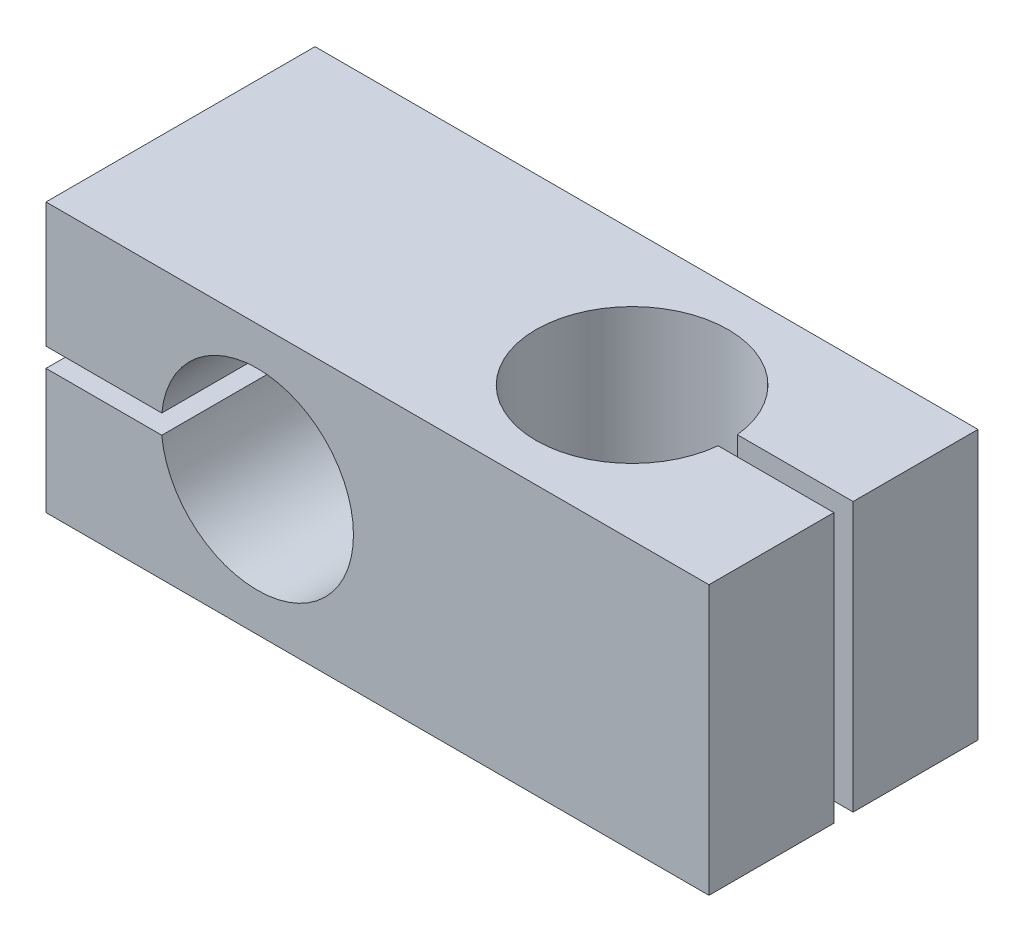
SolidWorks part; units mm, degrees
material "厂家标准"
ref_plane "前视基准面" through (0, 0, 0) normal (0, 0, 1) x (1, 0, 0)
ref_plane "上视基准面" through (0, 0, 0) normal (0, 1, 0) x (1, 0, 0)
ref_plane "右视基准面" through (0, 0, 0) normal (1, 0, 0) x (0, 0, -1)
sketch "草图1" plane through (0, 0, 0) normal (0, 0, 1) x (1, 0, 0)
  line L1 (-34.5, 14) -> (34.5, 14)
  line L2 (-34.5, 14) -> (-34.5, -14)
  line L3 (-34.5, -14) -> (34.5, -14)
  line L4 (34.5, 14) -> (34.5, -14)
  line L5 (-34.5, 14) -> (34.5, -14) construction
  line L6 (-34.5, -14) -> (34.5, 14) construction
  point P0 (0, 0)
  dimension "A" = 69
  dimension "B" = 28
extrude "凸台-拉伸1" add sketch "草图1" along normal mid plane 28
sketch "草图2" plane through (0, 0, 14) normal (0, 0, 1) x (1, 0, 0)
  line L0 (-34.5, 14) -> (-34.5, -14) construction
  line L1 (-34.5, 1) -> (-22.4499, 1)
  line L2 (-34.5, 1) -> (-34.5, -1)
  line L3 (-34.5, -1) -> (-22.4499, -1)
  line L4 (0, 14) -> (0, -14) construction
  line L5 (34.5, 14) -> (-34.5, 14) construction
  line L6 (-34.5, -14) -> (34.5, -14) construction
  arc A0 (-22.4499, -1) -> (-22.4499, 1) centre (-12.5, 0) ccw
extrude "切除-拉伸1" cut sketch "草图2" against normal through all
sketch "草图3" plane through (0, 14, 0) normal (0, 1, 0) x (1, 0, 0)
  line L0 (0, -14) -> (0, 14) construction
  line L1 (34.5, -14) -> (-34.5, -14) construction
  line L2 (34.5, 14) -> (-34.5, 14) construction
  line L3 (34.5, -14) -> (34.5, 14) construction
  line L4 (22.4499, -1) -> (34.5, -1)
  line L6 (22.4499, 1) -> (34.5, 1)
  line L7 (34.5, -1) -> (34.5, 1)
  arc A0 (22.4499, 1) -> (22.4499, -1) centre (12.5, 0) ccw
extrude "切除-拉伸2" cut sketch "草图3" against normal through all
equation "\"D3@草图3\"=\"F@草图2\""
equation "\"D1@草图3\"=\"D@草图2\""
equation "\"D2@草图3\"=\"D1@草图2\""
